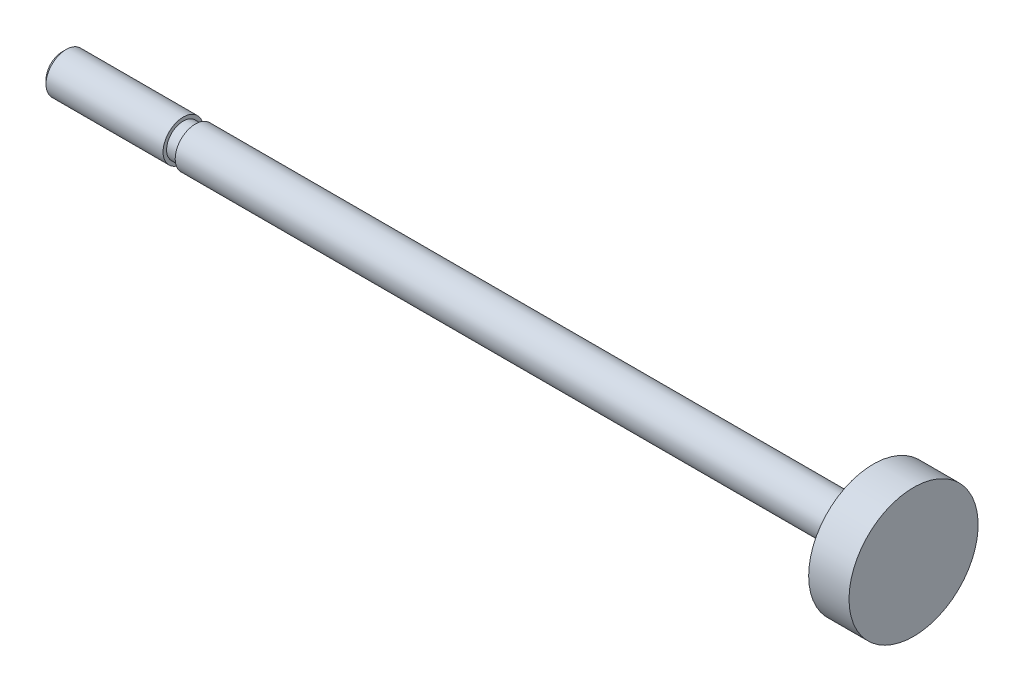
from build123d import *


with BuildPart() as part:
    # 草图1 → 旋转1 (revolve)
    with BuildSketch(Plane.XY, mode=Mode.PRIVATE) as revolve_1_sk:
        Polygon((0, 0), (0, 2.0095), (0.4905, 2.5), (15, 2.5), (15, 2.065), (16.5, 2.065), (16.5, 2.5), (100.5, 2.5), (100.5, 8), (105.5, 8), (105.5, 0), align=None)
    revolve(revolve_1_sk.sketch.rotate(Axis((105.5, 0, 0), (-1, 0, 0)), 270), axis=Axis((105.5, 0, 0), (-1, 0, 0)))


solid = part.part
